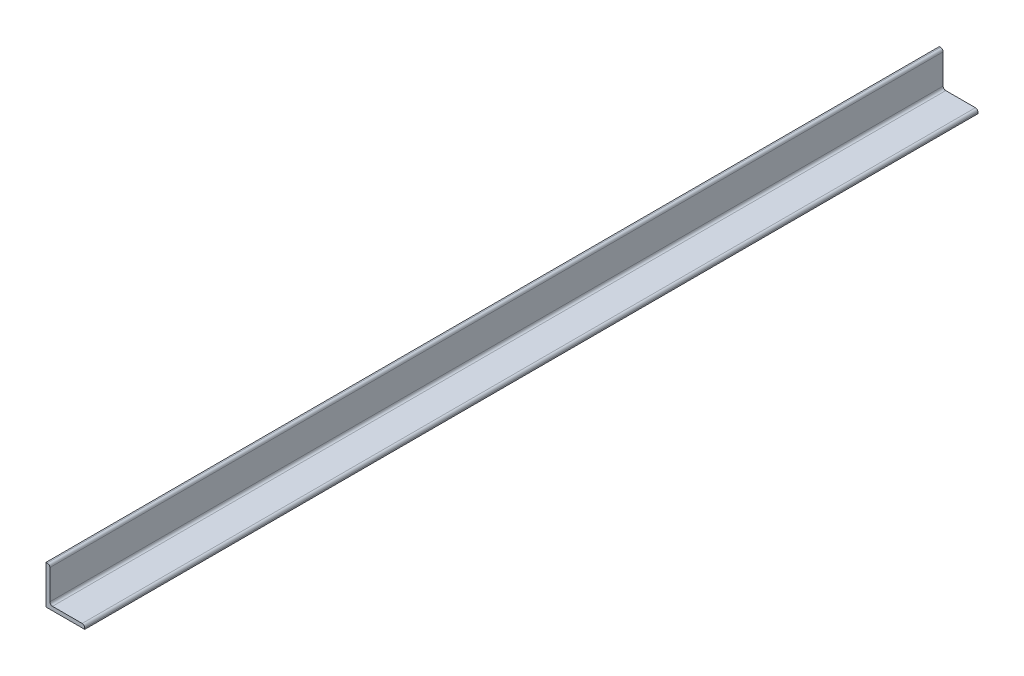
SolidWorks part; units mm, degrees
material "Plain Carbon Steel"
ref_plane "Front Plane" through (0, 0, 0) normal (0, 0, 1) x (1, 0, 0)
ref_plane "Top Plane" through (0, 0, 0) normal (0, 1, 0) x (1, 0, 0)
ref_plane "Right Plane" through (0, 0, 0) normal (1, 0, 0) x (0, 0, -1)
sketch "Sketch1" plane through (0, 0, 0) normal (0, 0, 1) x (1, 0, 0)
  line L0 (0, 0) -> (30, 0)
  line L1 (0, 0) -> (0, 30)
  line L2 (5, 3) -> (28, 3)
  line L3 (3, 5) -> (3, 28)
  line L4 (0, 30) -> (1, 30)
  line L5 (30, 1) -> (30, 0)
  line L6 (3, 3) -> (30, 3) construction
  line L7 (3, 3) -> (3, 30) construction
  arc A0 (30, 1) -> (28, 3) centre (28, 1) ccw
  arc A1 (5, 3) -> (3, 5) centre (5, 5) cw
  arc A2 (3, 28) -> (1, 30) centre (1, 28) ccw
  dimension "D4" = 2
  dimension "D1" = 30
  dimension "D2" = 30
  dimension "D3" = 3
extrude "Boss-Extrude1" add sketch "Sketch1" along normal blind 692
sketch "Sketch3" plane through (0, 0, 692) normal (0, 0, 1) x (1, 0, 0)
  line L1 (0, 30) -> (5, 30)
  line L2 (0, 30) -> (0, 3)
  line L3 (0, 3) -> (5, 3)
  line L4 (5, 30) -> (5, 3)
